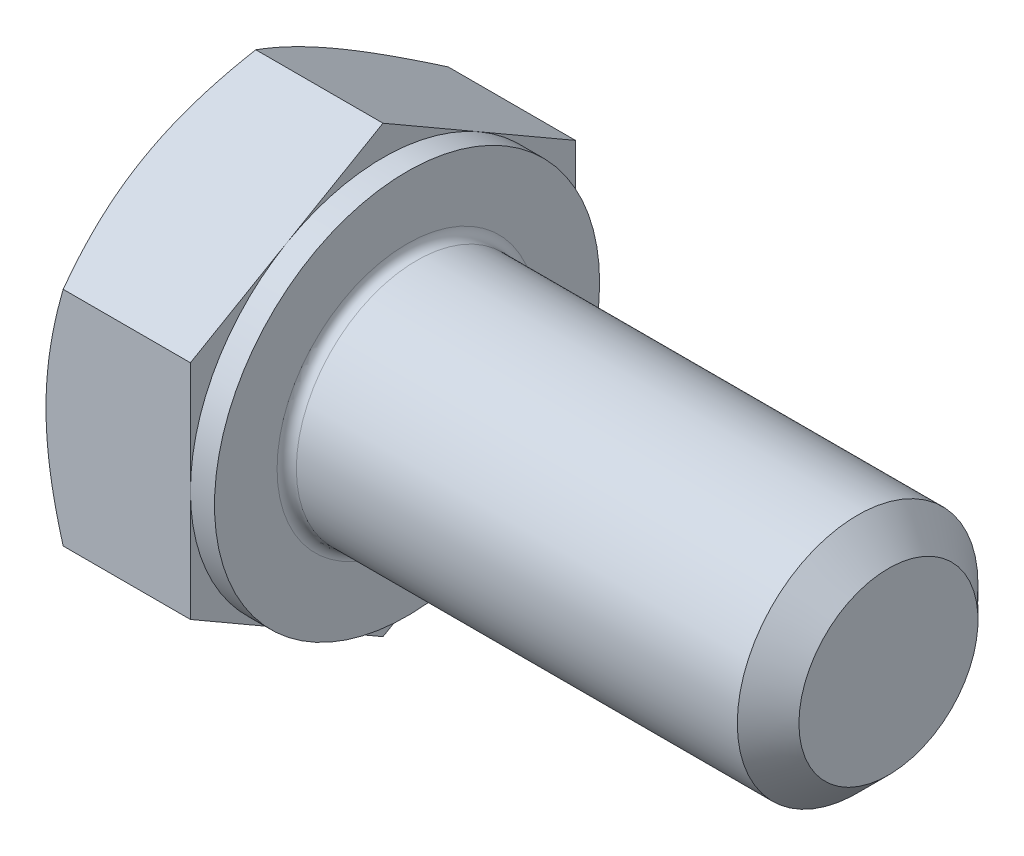
SolidWorks part; units mm, degrees
extrude "Base-Extrude" add sketch "Sketch1" along normal blind 3.5
sketch "Sketch1" plane through (0, 0, 0) normal (1, 0, 0) x (0, 0, -1)
  line L0 (4, 2.3094) -> (4, -2.3094)
  line L1 (-4, 2.3094) -> (-4, -2.3094)
  line L2 (4, -2.3094) -> (0, -4.6188)
  line L3 (0, -4.6188) -> (-4, -2.3094)
  line L4 (4, 2.3094) -> (0, 4.6188)
  line L5 (0, 4.6188) -> (-4, 2.3094)
revolve "Cut-Revolve1" cut sketch "Sketch3" angle 360 about L6
sketch "Sketch3" plane through (0, 0, 0) normal (0, 0, 1) x (1, 0, 0)
  line L0 (0, 4) -> (3.244, 9.6188)
  line L1 (0, 4.6188) -> (0, 2.3094) construction
  line L2 (3.244, 9.6188) -> (3.244, 14.6188)
  line L3 (3.244, 14.6188) -> (-10, 14.6188)
  line L4 (-10, 14.6188) -> (-10, 4)
  line L5 (-10, 4) -> (0, 4)
  line L6 (0, 0) -> (99.06, 0) construction
  line L7 (3.5, 4.6188) -> (0, 4.6188) construction
revolve "Boss-Revolve1" add sketch "Sketch2" angle 360 about L7
sketch "Sketch2" plane through (0, 0, 0) normal (0, 0, 1) x (1, 0, 0)
  line L0 (0, 2.3094) -> (0, -2.3094) construction
  line L1 (0, 0) -> (13.5, 0)
  line L2 (0, 0) -> (0, 2.5)
  line L3 (0, 2.5) -> (13.5, 2.5)
  line L4 (13.5, 0) -> (13.5, 1.8072)
  line L5 (3.5, 4.6188) -> (3.5, 2.3094) construction
  line L7 (0, 0) -> (96.52, 0) construction
  line L8 (13.5, -1.8072) -> (90.335, -2.5) construction
  line L9 (0, -2.5) -> (90.335, -2.5) construction
  line L10 (4.3, 15.24) -> (4.3, -1.27) construction
  line L11 (3.5, 15.24) -> (3.5, -1.27) construction
  line L12 (3.5, 2.3094) -> (3.5, -2.3094) construction
  line L14 (13.5, 2.5) -> (13.5, 1.8072)
  dimension "l" = 10
  dimension "m" = 5
  dimension "Minor_dia" = 3.6144
  dimension "p" = 0.8
  dimension "h" = 10
cosmetic thread "Helix1" parameters "Thread_length"=9.2, "Thread_minor"=3.6144
material "3.6级"
ref_plane "Front Plane" through (0, 0, 0) normal (0, 0, 1) x (1, 0, 0)
ref_plane "Top Plane" through (0, 0, 0) normal (0, 1, 0) x (1, 0, 0)
ref_plane "Right Plane" through (0, 0, 0) normal (1, 0, 0) x (0, 0, -1)
sketch "Sketch5" plane through (0, 0, 0) normal (0, 0, 1) x (1, 0, 0)
  line L0 (3.5, 4) -> (0.256, 9.6188)
  line L1 (3.5, 4.6188) -> (3.5, 2.3094) construction
  line L2 (0.256, 9.6188) -> (0.256, 14.6188)
  line L3 (0.256, 14.6188) -> (10.256, 14.6188)
  line L4 (10.256, 14.6188) -> (10.256, 4)
  line L5 (10.256, 4) -> (3.5, 4)
  line L7 (3.5, 4.6188) -> (0.3573, 4.6188) construction
  line L8 (0, 0) -> (99.06, 0) construction
  line L9 (0, 0) -> (99.06, 0) construction
revolve "Cut-Revolve2" cut sketch "Sketch5" angle 360 about L8
sketch "Sketch4" plane through (0, 0, 0) normal (0, 0, 1) x (1, 0, 0)
  line L1 (3.5, 4.6188) -> (3.5, 2.3094) construction
  line L2 (3.5, 4) -> (3, 4)
  line L3 (3.5, 4) -> (3.5, 14.6188)
  line L4 (3.5, 14.6188) -> (3, 14.6188)
  line L5 (0, 0) -> (95.25, 0) construction
  line L6 (0, 0) -> (96.52, 0) construction
  line L7 (3, 4) -> (3, 14.6188)
  line L8 (3.1427, 4.6188) -> (0.3573, 4.6188) construction
revolve "Cut-Revolve3" cut sketch "Sketch4" angle 360 about L5
chamfer "Chamfer" distance 0.64 angle 45 1 edges at (13.5, 0, 2.5)
fillet "Fillet" radius 0.2 1 edges at (3.5, 0, -2.5)
sketch "Sketch6" plane through (0, 0, 0) normal (0, 0, 1) x (1, 0, 0)
  line L0 (4.1, -1.8072) -> (3.7, -2.5)
  line L1 (4.1, -1.8072) -> (4.5, -2.5)
  line L2 (4.5, -2.5) -> (4.5, -3.125)
  line L3 (-3.175, 0) -> (5.1513, 0) construction
  line L5 (4.5, -3.125) -> (3.7, -3.125)
  line L6 (3.7, -3.125) -> (3.7, -2.5)
  arc A0 (3.7, -2.5) -> (3.5, -2.7) centre (3.7, -2.7) ccw construction
revolve "Cut-Revolve4" [suppressed] cut sketch "Sketch6" angle 360 about L3
pattern_linear "LPattern1" [suppressed]
equation "\"D3@Sketch1\" = \"s@Sketch1\" / 2"
equation "\"D4@Sketch1\" = \"D3@Sketch1\""
equation "\"D5@Sketch1\" = \"D4@Sketch1\""
equation "\"D1@Sketch3\" = \"s@Sketch1\" / 2"
equation "\"D1@Sketch5\" = \"s@Sketch1\" / 2"
equation "\"Head_ch_ang@Sketch5\" = \"Head_ch_ang@Sketch3\""
equation "\"D1@Sketch4\" = \"s@Sketch1\""
equation "\"Diameter@Sketch6\" = \"m@Sketch2\""
equation "\"Overcut@Sketch6\" = \"m@Sketch2\" * 1.25"
equation "\"Minor_dia@Sketch2\" = \"m@Sketch2\"-\"p@Sketch2\" * 1.732"
equation "\"Thread_minor@Helix1\" = \"Minor_dia@Sketch2\""
equation "\"Thread_minor@Sketch6\" = \"Minor_dia@Sketch2\""
equation "\"D1@Chamfer\" = \"p@Sketch2\"*0.8"
equation "\"Thread_length@Helix1\" = \"l@Sketch2\" - \"p@Sketch2\""
equation "\"Num_threads@LPattern1\" = \"l@Sketch2\" / \"p@Sketch2\""
